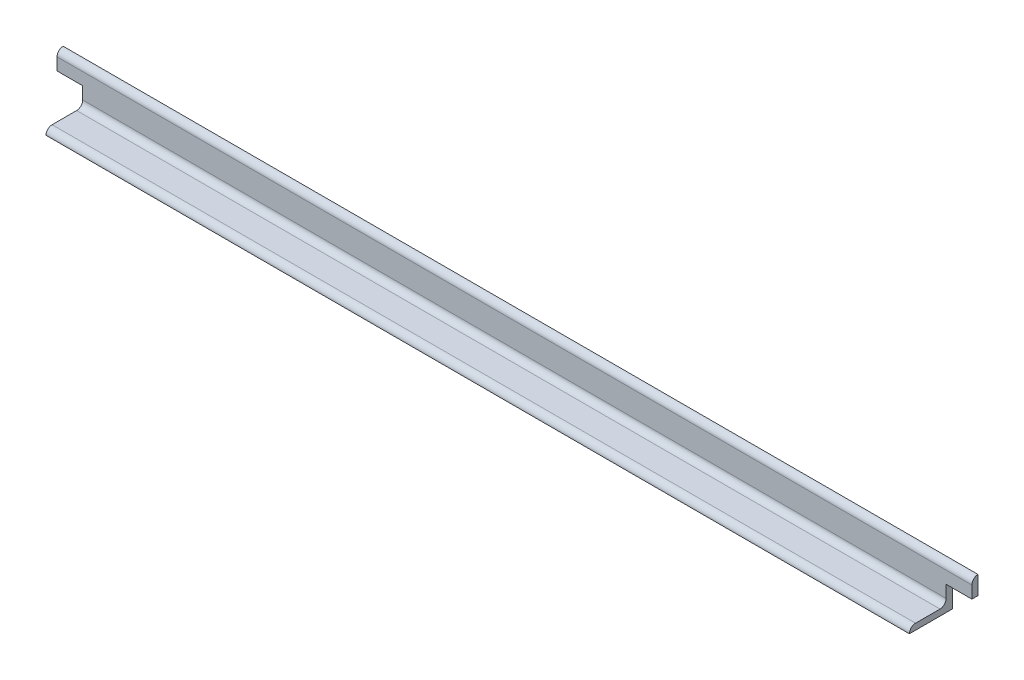
from build123d import *

# Parameters (mm, degrees)
ANGLE_IRON_35_X_35_X_5_1_DEPTH = 747
SKETCH2_W                      = 21
SKETCH2_H                      = 20
CUT_EXTRUDE1_DEPTH             = 749.638096813


with BuildPart() as part:
    # Sketch11 → Angle Iron 35 X 35 X 5(1) (new body)
    with BuildSketch(Plane.YZ):
        with BuildLine():
            Line((0, 0), (0, 35))
            ThreePointArc((0, 35), (3.535533906, 33.535533906), (5, 30))
            Line((5, 30), (5, 10))
            ThreePointArc((5, 10), (6.464466094, 6.464466094), (10, 5))
            Line((10, 5), (30, 5))
            ThreePointArc((30, 5), (33.535533906, 3.535533906), (35, 0))
            Line((35, 0), (0, 0))
        make_face()
    extrude(amount=ANGLE_IRON_35_X_35_X_5_1_DEPTH)

    # Sketch2 → Cut-Extrude1 (cut, through all)
    with BuildSketch(Plane(origin=(0, 0, 0), x_dir=(-1, 0, 0), z_dir=(0, 0, -1))):
        with Locations((-10.5, 10)):
            Rectangle(SKETCH2_W, SKETCH2_H)
        with Locations((-736.5, 10)):
            Rectangle(SKETCH2_W, SKETCH2_H)
    extrude(amount=-CUT_EXTRUDE1_DEPTH, mode=Mode.SUBTRACT)


solid = part.part
